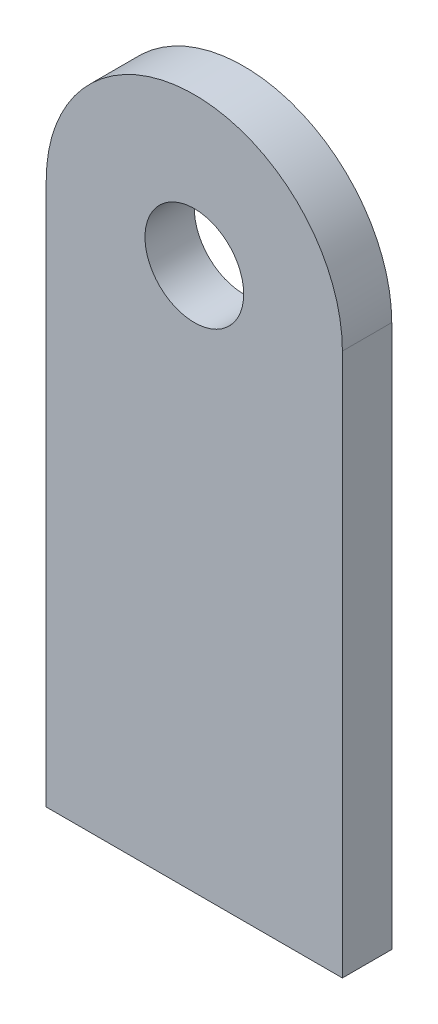
from build123d import *

# Parameters (mm, degrees)
SKETCH_1_R      = 5
EXTRUDE_1_DEPTH = 5


with BuildPart() as part:
    # 草图1 → 凸台-拉伸1 (new body)
    with BuildSketch(Plane.XY):
        with BuildLine():
            Line((0, 0), (30, 0))
            Line((30, 0), (30, 55))
            ThreePointArc((30, 55), (15, 70), (0, 55))
            Line((0, 55), (0, 0))
        make_face()
        with Locations((15, 55)):
            Circle(SKETCH_1_R, mode=Mode.SUBTRACT)
    extrude(amount=EXTRUDE_1_DEPTH)


solid = part.part
